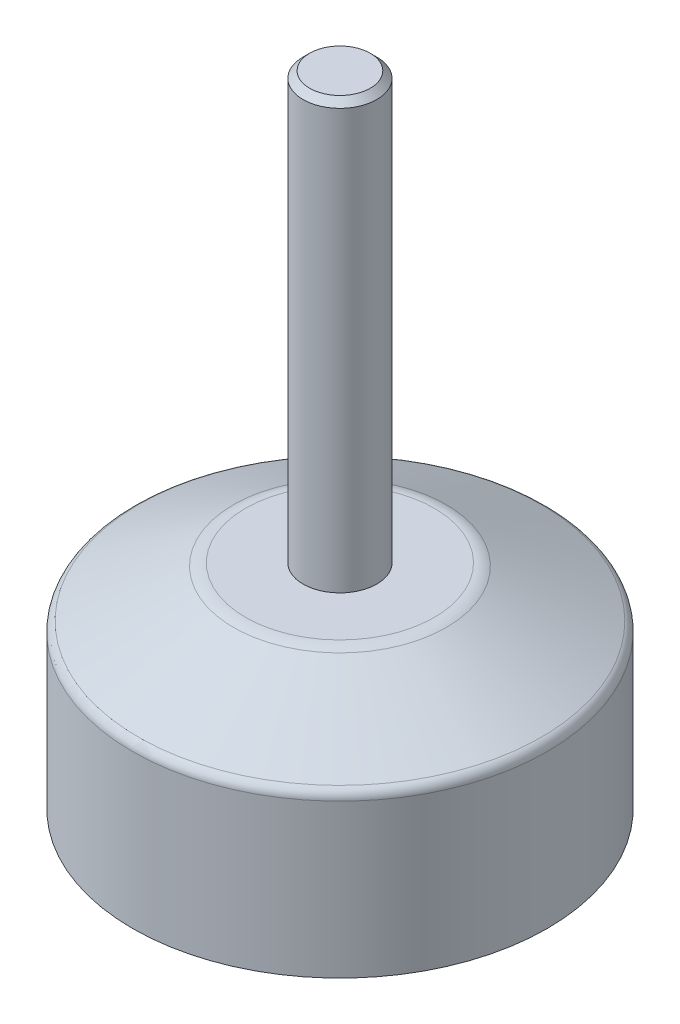
from build123d import *


with BuildPart() as part:
    # 草图1 → 旋转1 (revolve)
    with BuildSketch(Plane(origin=(0, 0, 0), x_dir=(-1, 0, 0), z_dir=(0, 0, -1)), mode=Mode.PRIVATE) as revolve_1_sk:
        with BuildLine():
            Line((-20, -25), (-0.54, -25))
            Line((-0.54, -25), (-0.54, 35))
            Line((-0.54, 35), (-3.3865, 35))
            Line((-3.3865, 35), (-4, 34.3865))
            Line((-4, 34.3865), (-4, -5))
            Line((-4, -5), (-9.409830056, -5))
            ThreePointArc((-9.409830056, -5), (-9.984212358, -5.066877526), (-10.527864045, -5.263932023))
            Line((-10.527864045, -5.263932023), (-19.447213595, -9.723606798))
            ThreePointArc((-19.447213595, -9.723606798), (-19.850650808, -10.092302877), (-20, -10.618033989))
            Line((-20, -10.618033989), (-20, -25))
        make_face()
    revolve(revolve_1_sk.sketch.rotate(Axis((0.54, -25, 0), (0, 1, 0)), 180), axis=Axis((0.54, -25, 0), (0, 1, 0)))


solid = part.part
